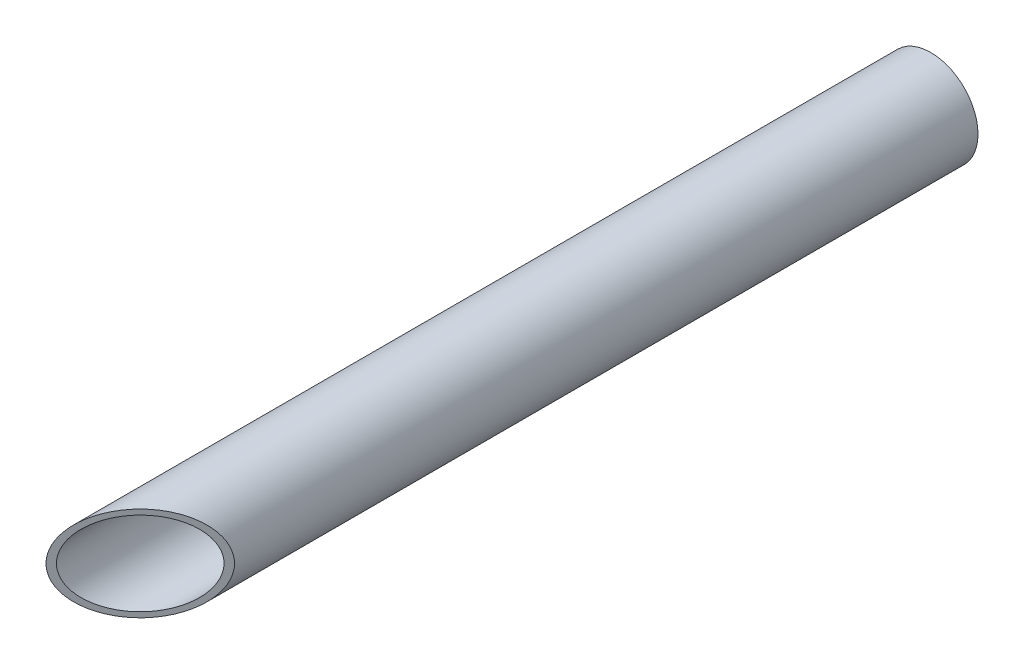
from build123d import *

# Parameters (mm, degrees)
SKETCH1_R           = 9
SKETCH1_R_2         = 8
BOSS_EXTRUDE1_DEPTH = 160
CUT_EXTRUDE1_DEPTH  = 80


with BuildPart() as part:
    # Sketch1 → Boss-Extrude1 (new body)
    with BuildSketch(Plane.XY):
        Circle(SKETCH1_R)
        Circle(SKETCH1_R_2, mode=Mode.SUBTRACT)
    extrude(amount=BOSS_EXTRUDE1_DEPTH)

    # Sketch2 → Cut-Extrude1 (cut, symmetric)
    with BuildSketch(Plane(origin=(0, 0, 0), x_dir=(1, 0, 0), z_dir=(0, 1, 0))):
        Polygon((-9, -160), (9, -142), (9, -160), align=None)
    extrude(amount=CUT_EXTRUDE1_DEPTH, both=True, mode=Mode.SUBTRACT)


solid = part.part
